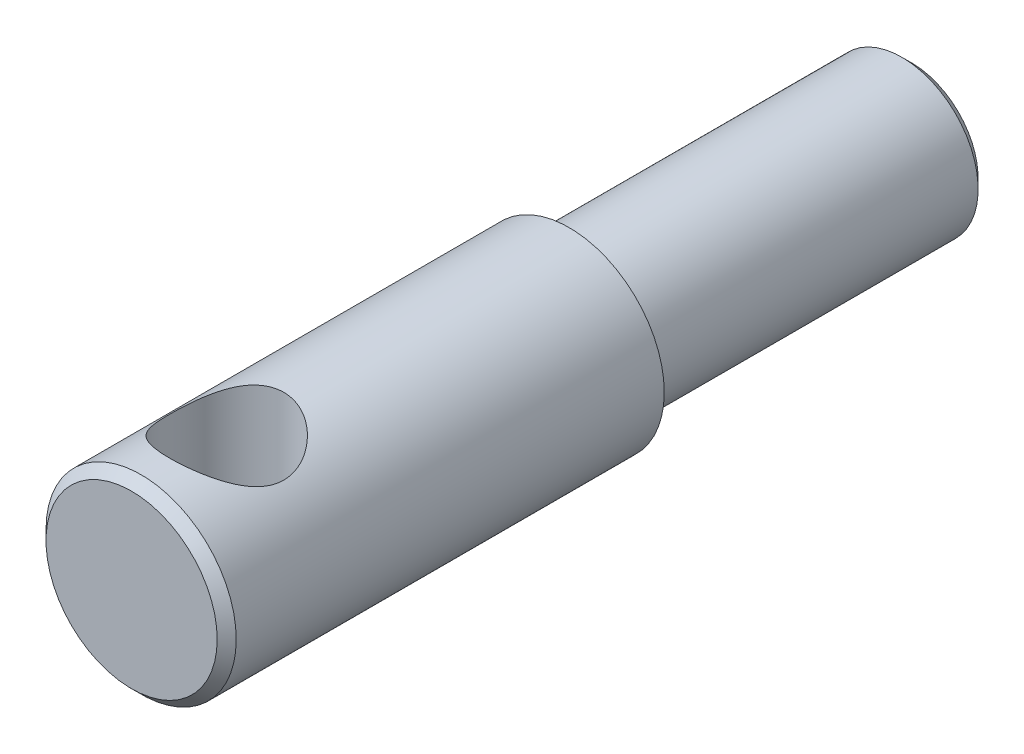
SolidWorks part; units mm, degrees
ref_plane "Front Plane" through (0, 0, 0) normal (0, 0, 1) x (1, 0, 0)
ref_plane "Top Plane" through (0, 0, 0) normal (0, 1, 0) x (1, 0, 0)
ref_plane "Right Plane" through (0, 0, 0) normal (1, 0, 0) x (0, 0, -1)
sketch "Sketch1" plane through (0, 0, 0) normal (0, 0, 1) x (1, 0, 0)
  circle A0 centre (0, 0) radius 5
  dimension "D1" = 10
extrude "Boss-Extrude1" add sketch "Sketch1" along normal blind 23
sketch "Sketch2" plane through (0, 0, 0) normal (0, 0, -1) x (-1, 0, 0)
  circle A0 centre (0, 0) radius 4
  dimension "D1" = 8
extrude "Boss-Extrude2" add sketch "Sketch2" along normal blind 18
cosmetic thread "Cosmetic Thread1" parameters "D2"=6.619
chamfer "Chamfer1" distance 0.5 angle 45 2 edges at (5, 0, 23) (-4, 0, -18)
sketch "Sketch3" plane through (0, 0, 0) normal (0, 1, 0) x (1, 0, 0)
  circle A0 centre (0, -18) radius 3
  dimension "D1" = 6
  dimension "D2" = 18
extrude "Cut-Extrude1" cut sketch "Sketch3" against normal through all both and the other way through all
